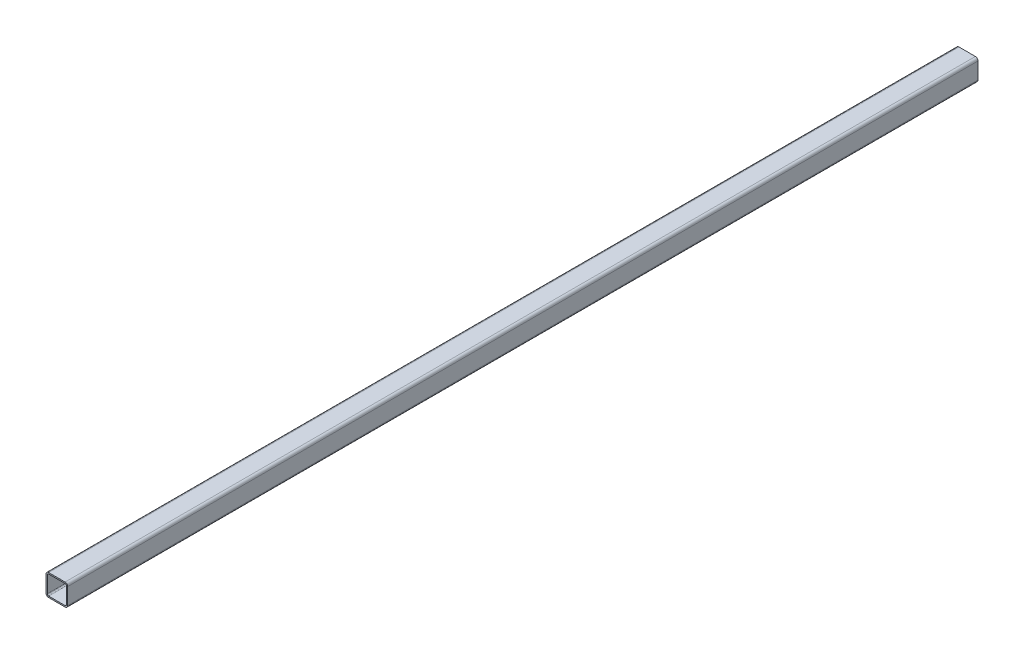
SolidWorks part; units mm, degrees
material "Q235B"
ref_plane "前视基准面" through (0, 0, 0) normal (0, 0, 1) x (1, 0, 0)
ref_plane "上视基准面" through (0, 0, 0) normal (0, 1, 0) x (1, 0, 0)
ref_plane "右视基准面" through (0, 0, 0) normal (1, 0, 0) x (0, 0, -1)
other "Configuration Table"
sketch "草图1" plane through (0, 0, 0) normal (1, 0, 0) x (0, 0, -1)
  line L0 (-1050, 0) -> (1050, 0)
other "Gb／6728-1986方形空心型钢 050 X 50 X 3(1)"
ref_plane "基准面1" through (0, 0, 1050) normal (0, 0, -1) x (0, 1, 0)
sketch "Sketch1" plane through (0, 0, 1050) normal (0, 0, -1) x (0, 1, 0)
  line L0 (-19, -22) -> (19, -22)
  line L1 (-22, -19) -> (-22, 19)
  line L2 (19, 22) -> (-19, 22)
  line L3 (22, 19) -> (22, -19)
  line L4 (-19, -25) -> (19, -25)
  line L5 (-25, -19) -> (-25, 19)
  line L6 (19, 25) -> (-19, 25)
  line L7 (25, 19) -> (25, -19)
  arc A0 (25, 19) -> (19, 25) centre (19, 19) ccw
  arc A1 (19, -25) -> (25, -19) centre (19, -19) ccw
  arc A2 (-25, -19) -> (-19, -25) centre (-19, -19) ccw
  arc A3 (-19, 25) -> (-25, 19) centre (-19, 19) ccw
  arc A4 (-19, 22) -> (-22, 19) centre (-19, 19) ccw
  arc A5 (22, 19) -> (19, 22) centre (19, 19) ccw
  arc A6 (19, -22) -> (22, -19) centre (19, -19) ccw
  arc A7 (-22, -19) -> (-19, -22) centre (-19, -19) ccw
  point P0 (-25, 0)
  point P1 (25, 0)
  point P2 (0, 25)
  point P3 (0, -25)
  point P4 (0, 0)
  point P5 (-25, -25)
  point P6 (25, -25)
  point P7 (25, 25)
  point P8 (-25, 25)
  point P33 (0, 0)
  dimension "D1" = 6
  dimension "Thickness" = 3
  dimension "V_leg" = 50
equation "\"D2@草图1\"=\"D1@草图1\"/2"
